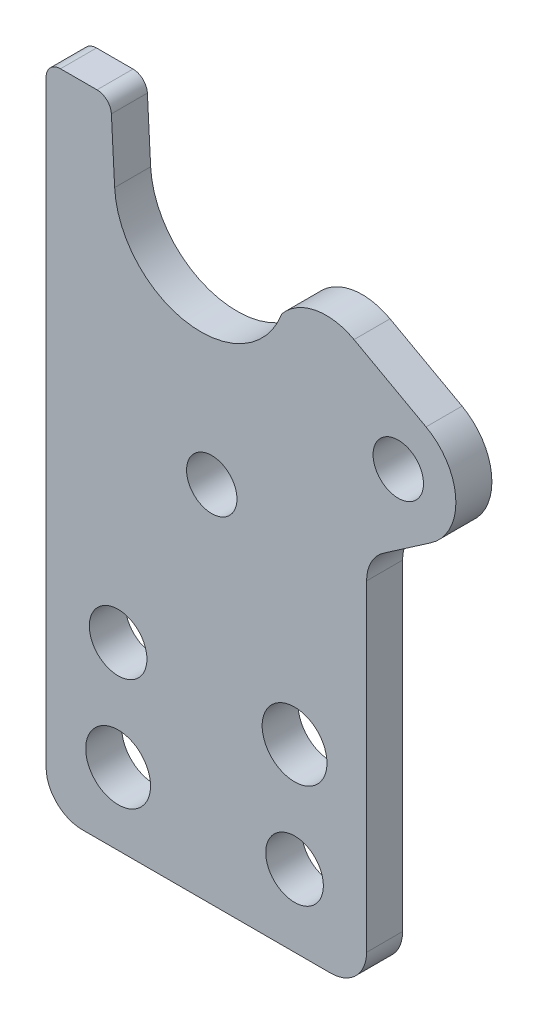
SolidWorks part; units mm, degrees
material "AISI 1045 钢，冷拔"
ref_plane "Front Plane" through (0, 0, 0) normal (0, 0, 1) x (1, 0, 0)
ref_plane "Top Plane" through (0, 0, 0) normal (0, 1, 0) x (1, 0, 0)
ref_plane "Right Plane" through (0, 0, 0) normal (1, 0, 0) x (0, 0, -1)
sketch "Sketch1" plane through (0, 0, 0) normal (0, 0, 1) x (1, 0, 0)
  line L0 (8.9647, 90) -> (9.5164, 79.472)
  line L1 (0, 0) -> (44.5, 0)
  line L2 (0, 0) -> (0, 90)
  line L3 (0, 90) -> (8.9647, 90)
  line L4 (44.5, 0) -> (44.5, 49.6662)
  line L5 (42.7553, 77.8097) -> (52.7553, 72.3097)
  line L6 (48.9, 72.3097) -> (48.9, 31.6389) construction
  line L7 (53.4373, 58.7111) -> (46.8806, 54.1961)
  arc A0 (9.5164, 79.472) -> (32.7448, 75.9101) centre (21.5, 80.1) ccw
  arc A1 (42.7553, 77.8097) -> (32.7448, 75.9101) centre (38.9, 70.8) ccw
  circle A2 centre (48.9, 65.3) radius 3.5
  arc A3 (53.4373, 58.7111) -> (52.7553, 72.3097) centre (48.9, 65.3) ccw
  arc A4 (46.8806, 54.1961) -> (44.5, 49.6662) centre (50, 49.6662) ccw
  circle A5 centre (10, 10) radius 4.5
  circle A6 centre (10, 25) radius 4
  circle A7 centre (34.5, 10) radius 4
  circle A8 centre (34.5, 25) radius 4.5
  circle A9 centre (23, 50.5) radius 3.5
  dimension "D3" = 21.5
  dimension "D4" = 9.9
  dimension "D6" = 24
  dimension "D7" = 38.9
  dimension "D8" = 19.2
  dimension "D9" = 48.9
  dimension "D10" = 24.7
  dimension "D11" = 7
  dimension "D12" = 16
  dimension "D13" = 8
  dimension "D14" = 50
  dimension "D16" = 11
  dimension "D17" = 10
  dimension "D18" = 10
  dimension "D19" = 10
  dimension "D20" = 15
  dimension "D21" = 9
  dimension "D22" = 8
  dimension "D23" = 9
  dimension "D24" = 8
  dimension "D25" = 10
  dimension "D26" = 10
  dimension "D27" = 10
  dimension "D28" = 15
  dimension "D29" = 7
  dimension "D30" = 23
  dimension "D31" = 50.5
  dimension "D1" = 44.5
  dimension "D2" = 90
  dimension "D5" = 93
  dimension "D15" = 34.552
extrude "Boss-Extrude1" add sketch "Sketch1" along normal blind 5
fillet "Fillet1" radius 2 2 edges at (8.9647, 90, 2.5) (0, 90, 2.5)
fillet "Fillet2" radius 5 2 edges at (44.5, 0, 2.5) (0, 0, 2.5)
